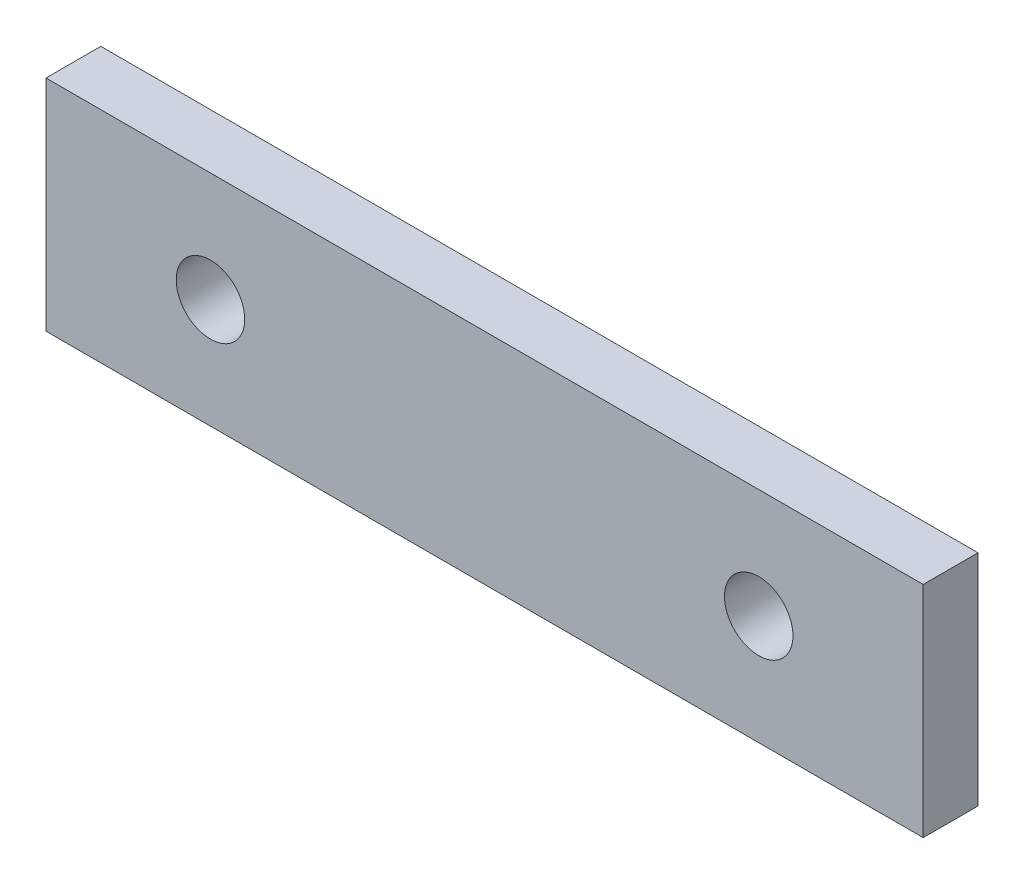
SolidWorks part; units mm, degrees
material "Q235B"
ref_plane "Front Plane" through (0, 0, 0) normal (0, 0, 1) x (1, 0, 0)
ref_plane "Top Plane" through (0, 0, 0) normal (0, 1, 0) x (1, 0, 0)
ref_plane "Right Plane" through (0, 0, 0) normal (1, 0, 0) x (0, 0, -1)
sketch "Sketch1" plane through (0, 0, 0) normal (0, 0, 1) x (1, 0, 0)
  line L1 (80, -20) -> (-80, -20)
  line L2 (80, -20) -> (80, 20)
  line L3 (80, 20) -> (-80, 20)
  line L4 (-80, -20) -> (-80, 20)
  line L5 (80, -20) -> (-80, 20) construction
  line L6 (80, 20) -> (-80, -20) construction
  point P0 (0, 0)
  dimension "D1" = 40
  dimension "D2" = 160
extrude "Boss-Extrude1" add sketch "Sketch1" along normal mid plane 10
hole_wizard "Ø12.5 (12.5) Diameter Hole1" positions "Sketch2" profile "Sketch3" hole size "Ø12.5" standard "GB" end condition through all
sketch "Sketch2" plane through (0, 0, 5) normal (0, 0, 1) x (1, 0, 0)
  line L0 (0, 20) -> (0, 0) construction
  line L1 (80, 20) -> (-80, 20) construction
  point P0 (-50, 0)
  point P12 (50, 0)
  dimension "D1" = 100
  dimension "D3" = 20
sketch "Sketch3" plane through (-50, 0, 5) normal (1, 0, 0) x (0, -1, 0)
  line L0 (0, 0) -> (0, 10)
  line L1 (0, 10) -> (6.25, 10)
  line L2 (6.25, 10) -> (6.25, 0)
  line L5 (6.25, 0) -> (0, 0)
  line L11 (0, -6.35) -> (0, 107.95) construction
  dimension "通孔孔直径" = 12.5
  dimension "通孔孔深度" = 10
hole_wizard "M8 Tapped Hole1" positions "Sketch4" profile "Sketch5" tap size "M8" standard "GB"
sketch "Sketch4" plane through (0, 0, 6) normal (0, 0, 1) x (1, 0, 0)
  line L0 (60, 235) -> (-60, 235) construction
  line L1 (0, 200) -> (0, 120) construction
  point P0 (0, 200)
  point P11 (0, 120)
  point P12 (0, 40)
  point P13 (0, -40)
  point P14 (0, -120)
  point P15 (0, -200)
  dimension "D1" = 35
  dimension "D3" = 80
  dimension "D2" = 6
sketch "Sketch5" plane through (0, 200, 6) normal (1, 0, 0) x (0, -1, 0)
  line L0 (0, 0) -> (0, 12)
  line L1 (0, 12) -> (3.4, 12)
  line L2 (3.4, 12) -> (3.4, 0)
  line L5 (3.4, 0) -> (0, 0)
  line L11 (0, -6.35) -> (0, 107.95) construction
  dimension "通孔螺纹孔钻头直径" = 6.8
  dimension "通孔螺纹孔钻头深度" = 12
cosmetic thread "Cosmetic Thread2" [suppressed] parameters "D2"=8
cosmetic thread "Cosmetic Thread3" [suppressed] parameters "D2"=8
cosmetic thread "Cosmetic Thread4" [suppressed] parameters "D2"=8
cosmetic thread "Cosmetic Thread5" [suppressed] parameters "D2"=8
cosmetic thread "Cosmetic Thread6" [suppressed] parameters "D2"=8
cosmetic thread "Cosmetic Thread7" [suppressed] parameters "D2"=8
